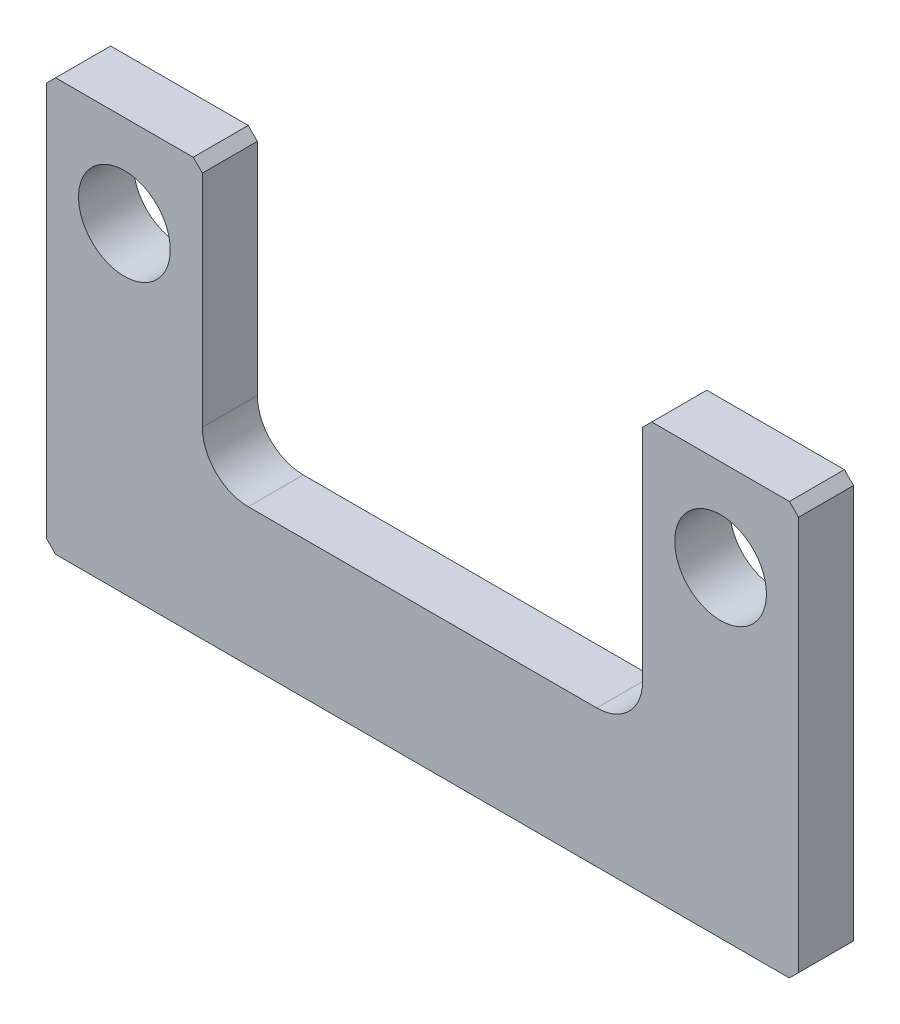
from build123d import *

# Parameters (mm, degrees)
SKETCH_1_R      = 10
EXTRUDE_1_DEPTH = 6
FILLET_1_R      = 10
CHAMFER_1_SIZE  = 2


with BuildPart() as part:
    # 草图1 → 凸台-拉伸1 (new, symmetric)
    with BuildSketch(Plane.XY):
        Polygon((-82, -70), (-82, 20), (-48, 20), (-48, -40), (48, -40), (48, 20), (82, 20), (82, -70), align=None)
        with Locations((-65, 0)):
            Circle(SKETCH_1_R, mode=Mode.SUBTRACT)
        with Locations((65, 0)):
            Circle(SKETCH_1_R, mode=Mode.SUBTRACT)
    extrude(amount=EXTRUDE_1_DEPTH, both=True)

    # 圆角1
    fillet_1_edges = [part.edges().sort_by_distance(p)[0] for p in [
        (-48, -40, 0),
        (48, -40, 0),
    ]]
    fillet(fillet_1_edges, radius=FILLET_1_R)

    # 倒角1
    chamfer_1_edges = [part.edges().sort_by_distance(p)[0] for p in [
        (-48, 20, 0),
        (48, 20, 0),
        (82, 20, 0),
        (82, -70, 0),
        (-82, -70, 0),
        (-82, 20, 0),
    ]]
    chamfer(chamfer_1_edges, length=CHAMFER_1_SIZE)


solid = part.part
